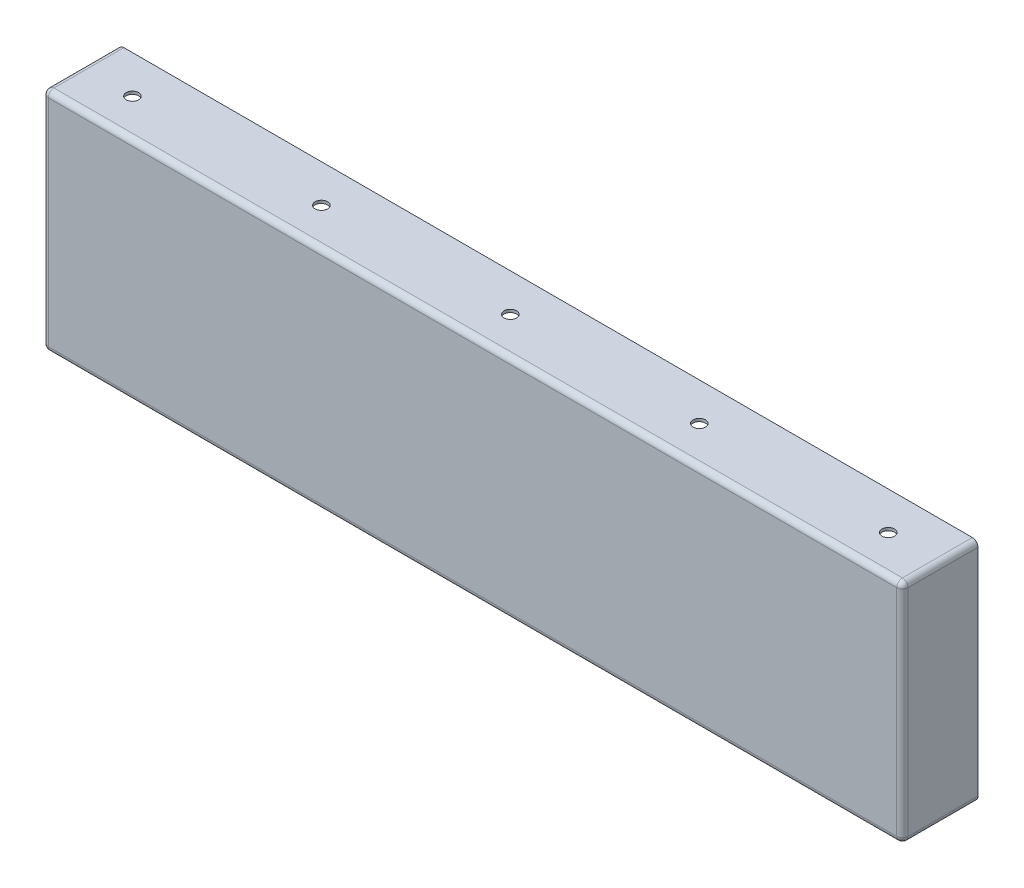
SolidWorks part; units mm, degrees
ref_plane "前视基准面" through (0, 0, 0) normal (0, 0, 1) x (1, 0, 0)
ref_plane "上视基准面" through (0, 0, 0) normal (0, 1, 0) x (1, 0, 0)
ref_plane "右视基准面" through (0, 0, 0) normal (1, 0, 0) x (0, 0, -1)
sketch "草图1" plane through (0, 0, 0) normal (0, 0, 1) x (1, 0, 0)
  line L1 (-227.5, -60) -> (227.5, -60)
  line L2 (-227.5, -60) -> (-227.5, 60)
  line L3 (-227.5, 60) -> (227.5, 60)
  line L4 (227.5, -60) -> (227.5, 60)
  line L5 (-227.5, -60) -> (227.5, 60) construction
  line L6 (-227.5, 60) -> (227.5, -60) construction
  point P0 (0, 0)
  dimension "D1" = 455
  dimension "D2" = 120
extrude "凸台-拉伸1" add sketch "草图1" along normal blind 40
fillet "圆角1" radius 3 8 edges at (227.5, -60, 20) (227.5, 60, 20) (227.5, 0, 40) (0, 60, 40) (-227.5, 60, 20) (-227.5, 0, 40) (0, -60, 40) (-227.5, -60, 20)
shell "抽壳1" thickness 1.5
hole_wizard "M6 间隙孔1" positions "草图2" profile "草图3" hole size "M6" standard "GB" end condition through all
sketch "草图2" plane through (0, -60, 0) normal (0, -1, 0) x (-1, 0, 0)
  line L0 (0, 0) -> (0, -40) construction
  line L1 (224.5, 0) -> (-224.5, 0) construction
  line L2 (224.5, -40) -> (-224.5, -40) construction
  point P0 (200, -20)
  point P2 (100, -20)
  point P4 (-100, -20)
  point P6 (-200, -20)
  point P17 (0, -20)
  dimension "D1" = 200
  dimension "D2" = 400
  dimension "D3" = 20
sketch "草图3" plane through (-200, -60, 20) normal (1, 0, 0) x (0, 0, -1)
  line L0 (0, 0) -> (0, 120)
  line L1 (0, 120) -> (3.3, 120)
  line L2 (3.3, 120) -> (3.3, 0)
  line L5 (3.3, 0) -> (0, 0)
  line L11 (0, -6.35) -> (0, 107.95) construction
  dimension "通孔孔直径" = 6.6
  dimension "通孔孔深度" = 120
